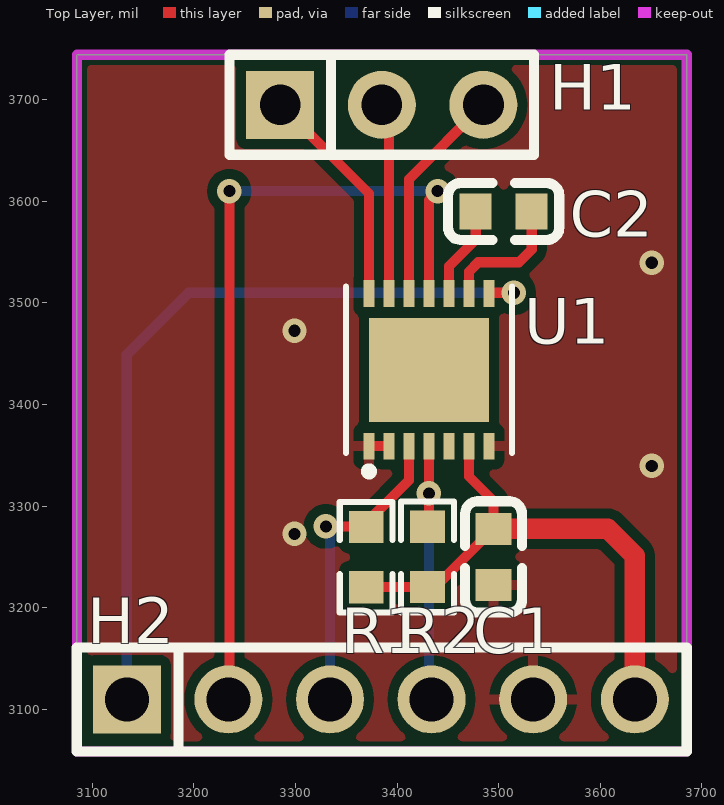
[diagram p0: Top Layer view]
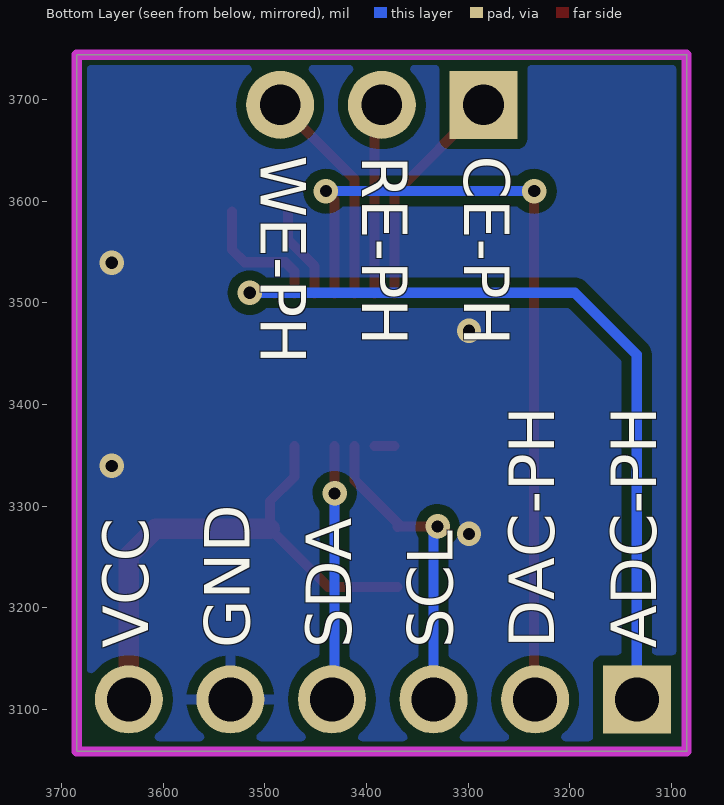
[diagram p1: Bottom Layer view, seen from below]
# Altium PCB MISC51980.pcbdoc
Units mil, origin at the board's own origin, x right, y up, seen from the top; angles counter-clockwise.
Board outline 600.2 x 685.66 mil, 2 copper layers (Top Layer, Bottom Layer), stack 62.206 mil thick; 7 components, 12 nets, 32 pads, 9 vias.

## Layer stack, top to bottom
Top Solder Mask Layer: solder mask 0.394, Dk 3.3
Top Layer: signal copper 1.379
Dielectric1: surface 59.449, FR4, Dk 4.5
Bottom Layer: signal copper 1.378
Bottom Solder Mask Layer: solder mask 0.394, Dk 3.3

## Board outline
3085,3744.21 3085,3058.55 3685.2,3058.55 3685.2,3744.21

## Design rules (kind name [scope] priority, off if disabled: settings)
BoardOutlineClearance copperThickness2oz_1 [All] p2 off: genericclearance=7.99 ignorepadtopadclearanceinfootprint=FALSE except(0: Arc-SplitContinuation Track-SplitContinuation SMDPad-SplitContinuation THPad-SplitContinuation Via-SplitContinuation Fill-SplitContinuation Region-SplitContinuation Poly-SplitContinuation Text-SplitContinuation Hole-SplitContinuation; 5.98: Arc-CutoutEdge SMDPad-CutoutEdge THPad-CutoutEdge Via-CutoutEdge Fill-CutoutEdge Region-CutoutEdge Text-CutoutEdge; 6.93: Hole-OutlineEdge Hole-CutoutEdge; 10: Poly-OutlineEdge Poly-CutoutEdge; 11.81: Arc-OutlineEdge Track-OutlineEdge SMDPad-OutlineEdge THPad-OutlineEdge Via-OutlineEdge Fill-OutlineEdge Region-OutlineEdge Text-OutlineEdge Track-CutoutEdge)
BoardOutlineClearance copperThickness1oz_1 [All] p4: genericclearance=4.02 ignorepadtopadclearanceinfootprint=FALSE except(0: Arc-SplitContinuation Track-SplitContinuation SMDPad-SplitContinuation THPad-SplitContinuation Via-SplitContinuation Fill-SplitContinuation Region-SplitContinuation Poly-SplitContinuation Text-SplitContinuation Hole-SplitContinuation; 6: SMDPad-CutoutEdge THPad-CutoutEdge Via-CutoutEdge Fill-CutoutEdge Region-CutoutEdge Text-CutoutEdge; 6.93: Hole-OutlineEdge Hole-CutoutEdge; 10: Poly-OutlineEdge Poly-CutoutEdge; 11.8: Arc-OutlineEdge Track-OutlineEdge SMDPad-OutlineEdge THPad-OutlineEdge Via-OutlineEdge Fill-OutlineEdge Region-OutlineEdge Text-OutlineEdge; 11.81: Arc-CutoutEdge Track-CutoutEdge)
Clearance copperThickness2oz [All] p1 off: gap=7.99 ignorepadtopadclearanceinfootprint=FALSE except(5.98: SMDPad-Track SMDPad-SMDPad THPad-Track SMDPad-THPad THPad-THPad Track-Via SMDPad-Via THPad-Via Via-Via Fill-Track Region-Track Fill-SMDPad Region-SMDPad Fill-THPad Region-THPad Fill-Via Region-Via Fill-Fill Fill-Region Region-Region Arc-Track Arc-SMDPad Arc-THPad Arc-Via Fill-Arc Region-Arc Arc-Arc Text-Track SMDPad-Text Text-THPad Text-Via Fill-Text Region-Text Arc-Text Text-Text; 6.93: Hole-Track Hole-SMDPad Hole-THPad Hole-Via Fill-Hole Region-Hole Hole-Arc Hole-Text; 10: Poly-Track Poly-SMDPad Poly-THPad Poly-Via Poly-Fill Poly-Region Poly-Poly Poly-Arc Poly-Text Poly-Hole)
Clearance copperThickness1oz [All] p3: gap=4.02 ignorepadtopadclearanceinfootprint=FALSE except(5.98: SMDPad-Track SMDPad-SMDPad THPad-Track SMDPad-THPad THPad-THPad Track-Via SMDPad-Via THPad-Via Via-Via Fill-Track Region-Track Fill-SMDPad Region-SMDPad Fill-THPad Region-THPad Fill-Via Region-Via Fill-Fill Fill-Region Region-Region; 6: Arc-Track Arc-SMDPad Arc-THPad Arc-Via Fill-Arc Region-Arc Arc-Arc Text-Track SMDPad-Text Text-THPad Text-Via Fill-Text Region-Text Arc-Text Text-Text; 6.93: Hole-Track Hole-SMDPad Hole-THPad Hole-Via Fill-Hole Region-Hole Hole-Arc Hole-Text; 10: Poly-Track Poly-SMDPad Poly-THPad Poly-Via Poly-Fill Poly-Region Poly-Poly Poly-Arc Poly-Text Poly-Hole)
Creepage creepage [All] p1: checkdistance=0 ignoreinternallayers=TRUE applytopolygonpour=TRUE
DiffPairsRouting differentialPair [All] p1: maxlimit=6 minlimit=6 mostfreqgap=6 toplayer_minwidth=5 toplayer_prefwidth=10 toplayer_maxwidth=100 toplayer_mingap=6 toplayer_prefgap=6 toplayer_maxgap=6 bottomlayer_minwidth=5 bottomlayer_prefwidth=10 bottomlayer_maxwidth=100 bottomlayer_mingap=6 bottomlayer_prefgap=6 bottomlayer_maxgap=6 maxuncoupledlength=10
HoleToHoleClearance otherClearance [All] p1: gap=11.81 allowstackedmicrovias=TRUE
Length netLength [All] p1: minlimit=0 maxlimit=0
MatchedLengths netLengthTolerance [All] p1: tolerance=1000
PasteMaskExpansion pasteMaskExpansion [All] p1: expansion=0
PlaneConnect innerPlane [All] p1: planeconnectstyle=Relief reliefexpansion=20 reliefentries=4 reliefconductorwidth=10 reliefairgap=10
PolygonConnect copperRegion [(InNet('GND'))] p1: connectstyle=Relief reliefconductorwidth=10 reliefentries=4 polygonreliefangle="90 Angle" airgapwidth=10 via.connectstyle=Relief via.reliefconductorwidth=10 via.reliefentries=4 via.polygonreliefangle="90 Angle" via.airgapwidth=10
RoutingVias viaSize [All] p1: holewidth=12.01 width=24.02 viastyle="Through Hole" minholewidth=11.81 minwidth=19.68 maxholewidth=248.03 maxwidth=393.7
SolderMaskExpansion solderMaskExpansion [IsVia] p1: expansion=-1000 istentingtop=TRUE
SolderMaskExpansion solderMaskExpansion [All] p2: expansion=2 istentingtop=FALSE
Width copperThickness2oz_2 [All] p1 off: maxlimit=100 minlimit=8 preferedwidth=10
Width copperThickness1oz_2 [All] p2: maxlimit=100 minlimit=5 preferedwidth=10

## Components (designator, comment, footprint, x,y, rotation, side; value= is the part's Value field where it differs from the comment)
C1 "100nF" C0603 3495,3250 r270 top
C2 "" C0603 3505,3590 r0 top
H1 "PZ254V-11-03P" HDR-TH_3P-P2.54-V-M_PZ254V-11-03P 3385,3695 r0 top
H2 "PZ254V-11-06P" HDR-TH_6P-P2.54-V-M 3384.02,3109.73 r0 top
R1 "4.7K" R0603 3369.66,3249.66 r270 top
R2 "4.7K" R0603 3430,3250 r270 top
U1 "LMP91000SDX/NOPB" WSON-14_L4.0-W4.0-P0.50-BL-EP-1 3431.43,3434.15 r0 top

## Footprints (in the part's own frame and the unit in brackets; to place one, negate y for a bottom-side part, rotate by r counter-clockwise, add the part's x,y. Pads: shape width x height; smd on the part's side, far side on the other; paste and mask are expansions set on the pad)
C0603 [mm]
  rect 0.8x0.9 smd: 1(-0.7,0) 2(0.7,0)
  silkscreen extent -1.39,-0.71 1.39,0.71
HDR-TH_3P-P2.54-V-M_PZ254V-11-03P [mm]
  rect 1.7x1.7 hole 1.02: 1(-2.54,0)
  round 1.7 hole 1.02: 2(0,0) 3(2.54,0)
  silkscreen extent -3.81,-1.25 3.81,1.25
HDR-TH_6P-P2.54-V-M [mm]
  rect 1.7x1.7 hole 1.1: 1(-6.35,0)
  round 1.7 hole 1.1: 2(-3.81,0) 3(-1.27,0) 4(1.27,0) 5(3.81,0) 6(6.35,0)
  silkscreen extent -7.6,-1.3 7.65,1.3
R0603 [mil]
  rect 31.75x34.02 smd paste-3937.01 mask+2: 1(-29.66,0) 2(29.66,0)
  silkscreen extent -55,-26 55,26
WSON-14_L4.0-W4.0-P0.50-BL-EP-1 [mm]
  rect 0.28x0.665 smd: 1(-1.5,-1.908) 2(-1,-1.908) 3(-0.5,-1.908) 4(0,-1.908) 5(0.5,-1.908) 6(1,-1.908) 7(1.5,-1.908) 8(1.5,1.908) 9(1,1.908) 10(0.5,1.908) 11(0,1.908) 12(-0.5,1.908) 13(-1,1.908) 14(-1.5,1.908)
  rect 3x2.6 smd: 15(0,0)
  silkscreen extent -2.08,-2.64 2.08,2.08

## Via types
v1: diameter 24.02, hole 12, Top Layer to Bottom Layer, 9 vias

## Nets (pads, with @x,y where several pads share a name; then routed paths per layer and width w, separated by ;. In a path a pad name is that pad's centre, name@x,y a point inside that pad or via, vN(x,y) a via of type N, cw(c..) or ccw(c..) an arc to the next point about the centre after c; other vN are vias at no path point)
$1N15: C2.2 U1.9 | length 129.8
  Top Layer w10: U1.9 3470.8,3530.8 3480,3540 3520,3540 3532.56,3552.56 C2.2
$1N17: C2.1 U1.10 | length 91.7
  Top Layer w10: U1.10 3451.12,3536.12 3477.44,3562.44 C2.1
ADC-PH: H2.1 U1.8 | length 770.4
  Top Layer w10: U1.8 3491.24,3510 v1(3515,3510)
  Bottom Layer w10: H2.1 3134.02,3449.02 3195,3510 v1(3515,3510)
CE-PH: H1.1 U1.14 | length 221.9
  Top Layer w10: H1.1 3372.38,3607.62 U1.14
DAC-PH: H2.2 U1.11 | length 810
  Top Layer w10: H2.2 3235,3110.72 v1(3235,3610) ; U1.11 3431.43,3601.43 v1(3440,3610)
  Bottom Layer w10: v1(3235,3610) v1(3440,3610)
GND: C1.2 H2.5 U1.1 U1.2 U1.7 | length 19.7
  Top Layer w10: U1.1 U1.2
  other v1: 3299.1,3272.65 3650.79,3339.52 3299.1,3472.65 3650.79,3539.52
RE-PH: H1.2 U1.13 | length 188.7
  Top Layer w10: H1.2 3392.06,3687.94 U1.13
SCL: H2.3 R1.1 U1.3 | length 309.7
  Top Layer w10: v1(3330,3280) R1.1@3366.41,3280 ; R1.1 3368.98,3280 R1.1@3366.41,3280 ; U1.3 3411.75,3325.34 R1.1@3366.41,3280
  Bottom Layer w10: v1(3330,3280) 3334.02,3275.98 H2.3
SDA: H2.4 R2.1 U1.4 | length 283.8
  Top Layer w10: R2.1 3431.43,3281.09 v1(3431.43,3312.5) U1.4
  Bottom Layer w10: v1(3431.43,3312.5) 3431.43,3112.32 H2.4
vcc: C1.1 H2.6 R1.2 R2.2 U1.6 | length 379.1
  Top Layer w10: R1.2@3369.66,3220.34 R2.2@3437.78,3220.34 ; 3470.8,3329.2 U1.6 ; C1.1 3495,3305
  Top Layer w20: C1.1 3607.44,3277.56 ; H2.6 3634.02,3250.98
VCC:  | length 152.7
  Top Layer w10: 3437.78,3220.34 3495,3277.56 ; 3470.8,3329.2 3495,3305
  Top Layer w20: 3607.44,3277.56 3634.02,3250.98
WE-PH: H1.3 U1.12 | length 216.1
  Top Layer w10: U1.12 3411.75,3621.75 H1.3
pads on no net: U1.5 U1.15

## Polygon pours and split planes (outlines as drawn)
GND on Top Layer (solid, remove dead copper, pour order 0): 3000,3810 3000,3000 3795,3000 3795,3810
GND on Bottom Layer (solid, remove dead copper, pour order 2): 3035,3810 3035,3005 3800,3005 3800,3810

## Keep-outs
Board Outline Layer:
  the board outline again, w10

## Silkscreen, mask and mechanical layers (free items; w line width, h text height)
Bottom Silkscreen Layer:
  text "CE-PH" at 3304.02,3644.73 h45 r90
  text "RE-PH" at 3404.02,3644.73 h45 r90
  text "WE-PH" at 3504.02,3644.73 h45 r90
  text "ADC-PH" at 3115,3160 h45 r270
  text "DAC-PH" at 3215,3160 h45 r270
  text "SCL" at 3315,3160 h45 r270
  text "SDA" at 3415,3160 h45 r270
  text "GND" at 3515,3160 h45 r270
  text "VCC" at 3615,3160 h45 r270